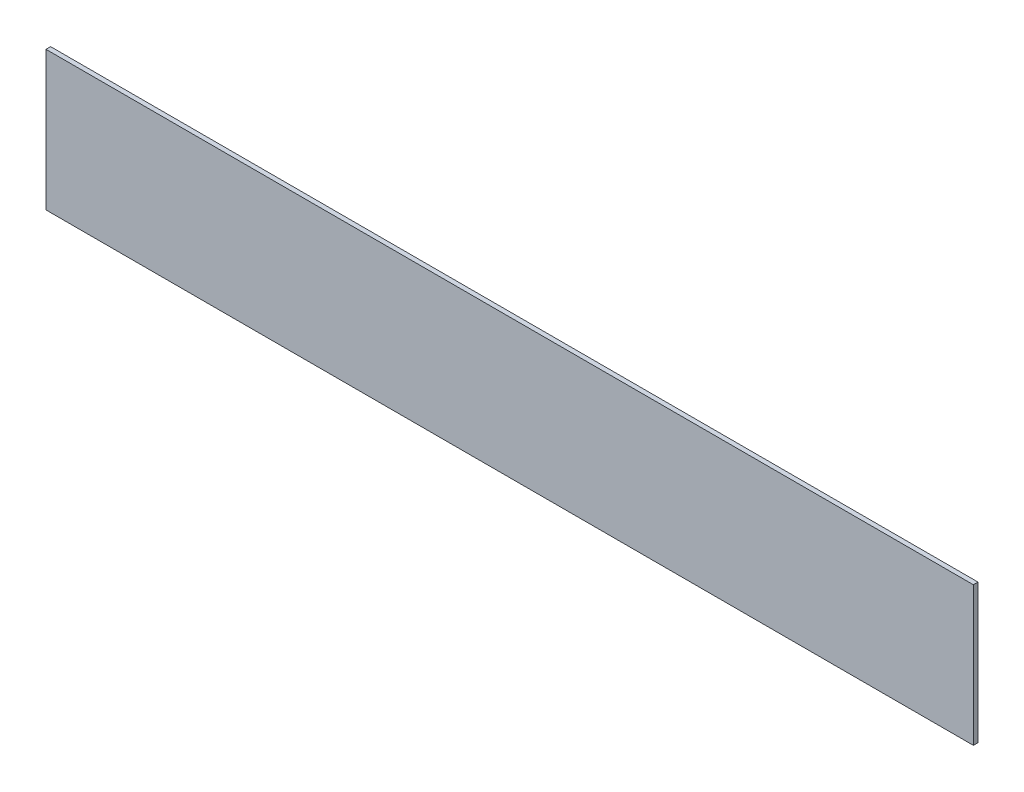
SolidWorks part; units mm, degrees
ref_plane "Front Plane" through (0, 0, 0) normal (0, 0, 1) x (1, 0, 0)
ref_plane "Top Plane" through (0, 0, 0) normal (0, 1, 0) x (1, 0, 0)
ref_plane "Right Plane" through (0, 0, 0) normal (1, 0, 0) x (0, 0, -1)
sketch "Sketch1" plane through (0, 0, 0) normal (0, 0, 1) x (1, 0, 0)
  line L1 (0, 0) -> (1000, 0)
  line L2 (0, 0) -> (0, 150)
  line L3 (0, 150) -> (1000, 150)
  line L4 (1000, 0) -> (1000, 150)
  dimension "D1" = 1000
  dimension "D2" = 150
extrude "Boss-Extrude1" add sketch "Sketch1" along normal blind 5
